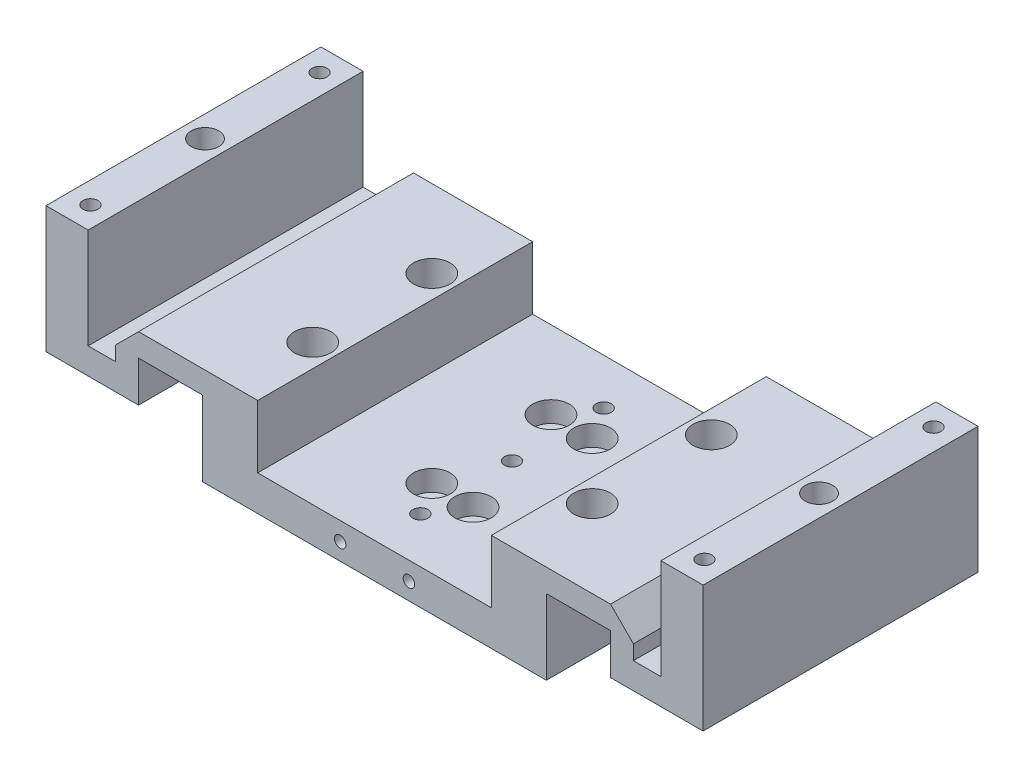
from build123d import *

# Parameters (mm, degrees)
EXTRUDE_1_DEPTH             = 30
CHAMFER_1_SIZE              = 5
SKETCH_2_R                  = 2
CUT_EXTRUDE_1_DEPTH         = 86.28129924
SKETCH_4_R                  = 3.5
CUT_EXTRUDE_3_DEPTH         = 4.5
SKETCH_5_R                  = 3.5
CUT_EXTRUDE_4_DEPTH         = 4.5
HOLE_WIZARD_M3_5_D          = 2.5
HOLE_WIZARD_M3_5_DEPTH      = 8.5
HOLE_WIZARD_M3_5_TIP        = 0.751075774
HOLE_WIZARD_M4_2_D          = 3.3
HOLE_WIZARD_2_D             = 4.5
HOLE_WIZARD_2_CBORE_D       = 8
HOLE_WIZARD_2_CBORE_DEPTH   = 6
HOLE_WIZARD_2_2_D           = 4.5
HOLE_WIZARD_2_2_CBORE_D     = 8
HOLE_WIZARD_2_2_CBORE_DEPTH = 4.5
PATTERN_LINEAR_1_COUNT      = 3
PATTERN_LINEAR_1_PITCH      = 20


with BuildPart() as part:
    # 草图1 → 凸台-拉伸1 (new, symmetric)
    with BuildSketch(Plane.XY):
        Polygon((37.5, 0), (-37.5, 0), (-37.5, 16.388182382), (-51.5, 16.388182382), (-51.5, 7.5), (-71.7, 7.5), (-71.7, 35.1), (-62.5, 35.1), (-62.5, 13.2), (-56.5, 13.2), (-56.5, 21.388182382), (-25.5, 21.388182382), (-25.5, 7.7), (25.5, 7.7), (25.5, 21.388182382), (56.5, 21.388182382), (56.5, 13.2), (62.5, 13.2), (62.5, 35.1), (71.7, 35.1), (71.7, 7.5), (51.5, 7.5), (51.5, 16.388182382), (37.5, 16.388182382), align=None)
    extrude(amount=EXTRUDE_1_DEPTH, both=True)

    # 倒角1
    chamfer_1_edges = [part.edges().sort_by_distance(p)[0] for p in [
        (-56.5, 21.388182382, 0),
        (56.5, 21.388182382, 0),
    ]]
    chamfer(chamfer_1_edges, length=CHAMFER_1_SIZE)

    # 草图2 → 切除-拉伸1 (cut, through all)
    with BuildSketch(Plane.XZ):
        with Locations(Location((-4.5, 13, 0), (0, 0, 270))):
            Circle(SKETCH_2_R)
        with Locations(Location((-30.5, 13, 0), (0, 0, 270))):
            Circle(SKETCH_2_R)
        with Locations(Location((30.5, 13, 0), (0, 0, 270))):
            Circle(SKETCH_2_R)
        with Locations(Location((4.5, 13, 0), (0, 0, 270))):
            Circle(SKETCH_2_R)
        with Locations(Location((4.5, -13, 0), (0, 0, 270))):
            Circle(SKETCH_2_R)
        with Locations(Location((30.5, -13, 0), (0, 0, 270))):
            Circle(SKETCH_2_R)
        with Locations(Location((-30.5, -13, 0), (0, 0, 270))):
            Circle(SKETCH_2_R)
        with Locations(Location((-4.5, -13, 0), (0, 0, 270))):
            Circle(SKETCH_2_R)
    extrude(amount=-CUT_EXTRUDE_1_DEPTH, mode=Mode.SUBTRACT)

    # 草图4 → 切除-拉伸3 (cut)
    with BuildSketch(Plane(origin=(0, 21.388182382, 0), x_dir=(1, 0, 0), z_dir=(0, 1, 0))):
        with Locations(Location((-30.5, 13, 0), (0, 0, 270))):
            Circle(SKETCH_4_R)
        with Locations(Location((-30.5, -13, 0), (0, 0, 270))):
            Circle(SKETCH_4_R)
        with Locations(Location((30.5, 13, 0), (0, 0, 270))):
            Circle(SKETCH_4_R)
        with Locations(Location((30.5, -13, 0), (0, 0, 270))):
            Circle(SKETCH_4_R)
    extrude(amount=-CUT_EXTRUDE_3_DEPTH, mode=Mode.SUBTRACT)

    # 草图5 → 切除-拉伸4 (cut)
    with BuildSketch(Plane(origin=(0, 7.7, 0), x_dir=(1, 0, 0), z_dir=(0, 1, 0))):
        with Locations(Location((-4.5, 13, 0), (0, 0, 270))):
            Circle(SKETCH_5_R)
        with Locations(Location((4.5, 13, 0), (0, 0, 270))):
            Circle(SKETCH_5_R)
        with Locations(Location((4.5, -13, 0), (0, 0, 270))):
            Circle(SKETCH_5_R)
        with Locations(Location((-4.5, -13, 0), (0, 0, 270))):
            Circle(SKETCH_5_R)
    extrude(amount=-CUT_EXTRUDE_4_DEPTH, mode=Mode.SUBTRACT)

    # 草图6 → M4 螺纹孔1 (revolve, cut)
    with BuildSketch(Plane(origin=(-67, 35.1, -25), x_dir=(0, 0, 1), z_dir=(1, 0, 0))):
        Polygon((0, 0), (0, 12.991420021), (1.65, 12), (1.65, 0), align=None)
    hole_wizard_m4_1 = revolve(axis=Axis((-67, 41.45, -25), (0, -1, 0)), mode=Mode.SUBTRACT)

    # 镜向1: M4 螺纹孔1 across plane
    add(hole_wizard_m4_1.mirror(Plane.XY), mode=Mode.SUBTRACT)

    # 镜向2: M4 螺纹孔1 across plane
    add(hole_wizard_m4_1.mirror(Plane(origin=(0, 0, 0), x_dir=(0, 0, 1), z_dir=(1, 0, 0))), mode=Mode.SUBTRACT)

    # 镜向2 copy 1 sketch → 镜向2 copy 1 (revolve, cut)
    with BuildSketch(Plane(origin=(67, 35.1, 25), x_dir=(0, 0, -1), z_dir=(-1, 0, 0))):
        Polygon((0, 0), (0, 12.991420021), (1.65, 12), (1.65, 0), align=None)
    revolve(axis=Axis((67, 41.45, 25), (0, -1, 0)), mode=Mode.SUBTRACT)

    # M3 螺纹孔5
    with Locations(Plane(origin=(0, 0, -30), x_dir=(-1, 0, 0), z_dir=(0, 0, -1))):
        with Locations((-33.5, 11), (-33.5, 17)):
            Hole(HOLE_WIZARD_M3_5_D / 2, depth=HOLE_WIZARD_M3_5_DEPTH)
            with Locations((0, 0, -(HOLE_WIZARD_M3_5_DEPTH + HOLE_WIZARD_M3_5_TIP / 2))):  # 118° drill point
                Cone(0, HOLE_WIZARD_M3_5_D / 2, HOLE_WIZARD_M3_5_TIP, mode=Mode.SUBTRACT)

    # M4 螺纹孔2 (through all)
    with Locations(Plane(origin=(0, 0, 0), x_dir=(-1, 0, 0), z_dir=(0, -1, 0))):
        with Locations((0, 20)):
            hole_wizard_m4_2 = Hole(HOLE_WIZARD_M4_2_D / 2)

    # 草图14 → M3 螺纹孔3 (revolve, cut)
    with BuildSketch(Plane(origin=(-7.5, 3.7, 30), x_dir=(0, -1, 0), z_dir=(1, 0, 0))):
        Polygon((0, 0), (0, 11.751075774), (1.25, 11), (1.25, 0), align=None)
    hole_wizard_m3_3 = revolve(axis=Axis((-7.5, 3.7, 36.35), (0, 0, -1)), mode=Mode.SUBTRACT)

    # 镜向4: M3 螺纹孔3 across plane
    add(hole_wizard_m3_3.mirror(Plane(origin=(0, 0, 0), x_dir=(0, 0, 1), z_dir=(1, 0, 0))), mode=Mode.SUBTRACT)

    # 镜向5: M3 螺纹孔3 across plane
    add(hole_wizard_m3_3.mirror(Plane.XY), mode=Mode.SUBTRACT)

    # 镜向5 copy 1 sketch → 镜向5 copy 1 (revolve, cut)
    with BuildSketch(Plane(origin=(7.5, 3.7, -30), x_dir=(0, -1, 0), z_dir=(-1, 0, 0))):
        Polygon((0, 0), (0, 11.751075774), (1.25, 11), (1.25, 0), align=None)
    revolve(axis=Axis((7.5, 3.7, -36.35), (0, 0, 1)), mode=Mode.SUBTRACT)

    # Hole Wizard 2 (through all)
    with Locations(Plane(origin=(0, 21.388182382, 0), x_dir=(1, 0, 0), z_dir=(0, 1, 0))):
        with Locations((-30.5, 13), (-30.5, -13), (30.5, 13), (30.5, -13)):
            CounterBoreHole(HOLE_WIZARD_2_D / 2, HOLE_WIZARD_2_CBORE_D / 2, HOLE_WIZARD_2_CBORE_DEPTH)

    # Hole Wizard 2 2 (through all)
    with Locations(Plane(origin=(0, 7.7, 0), x_dir=(1, 0, 0), z_dir=(0, 1, 0))):
        with Locations((-4.5, 13), (4.5, 13), (-4.5, -13), (4.5, -13)):
            CounterBoreHole(HOLE_WIZARD_2_2_D / 2, HOLE_WIZARD_2_2_CBORE_D / 2, HOLE_WIZARD_2_2_CBORE_DEPTH)

    # 阵列(线性)1: M4 螺纹孔2 ×3
    with Locations(*[(0, 0, i * PATTERN_LINEAR_1_PITCH) for i in range(1, PATTERN_LINEAR_1_COUNT)]):
        add(hole_wizard_m4_2, mode=Mode.SUBTRACT)

    # 草图22 → 大小mm 暗销孔1 (revolve, cut)
    with BuildSketch(Plane(origin=(67, 35.1, 0), x_dir=(0, 0, 1), z_dir=(1, 0, 0))):
        Polygon((0, 0), (0, 16.802581857), (3, 15), (3, 0), align=None)
    mm_1 = revolve(axis=Axis((67, 41.45, 0), (0, -1, 0)), mode=Mode.SUBTRACT)

    # 镜向6: 大小mm 暗销孔1 across plane
    add(mm_1.mirror(Plane(origin=(0, 0, 0), x_dir=(0, 0, 1), z_dir=(1, 0, 0))), mode=Mode.SUBTRACT)


solid = part.part
